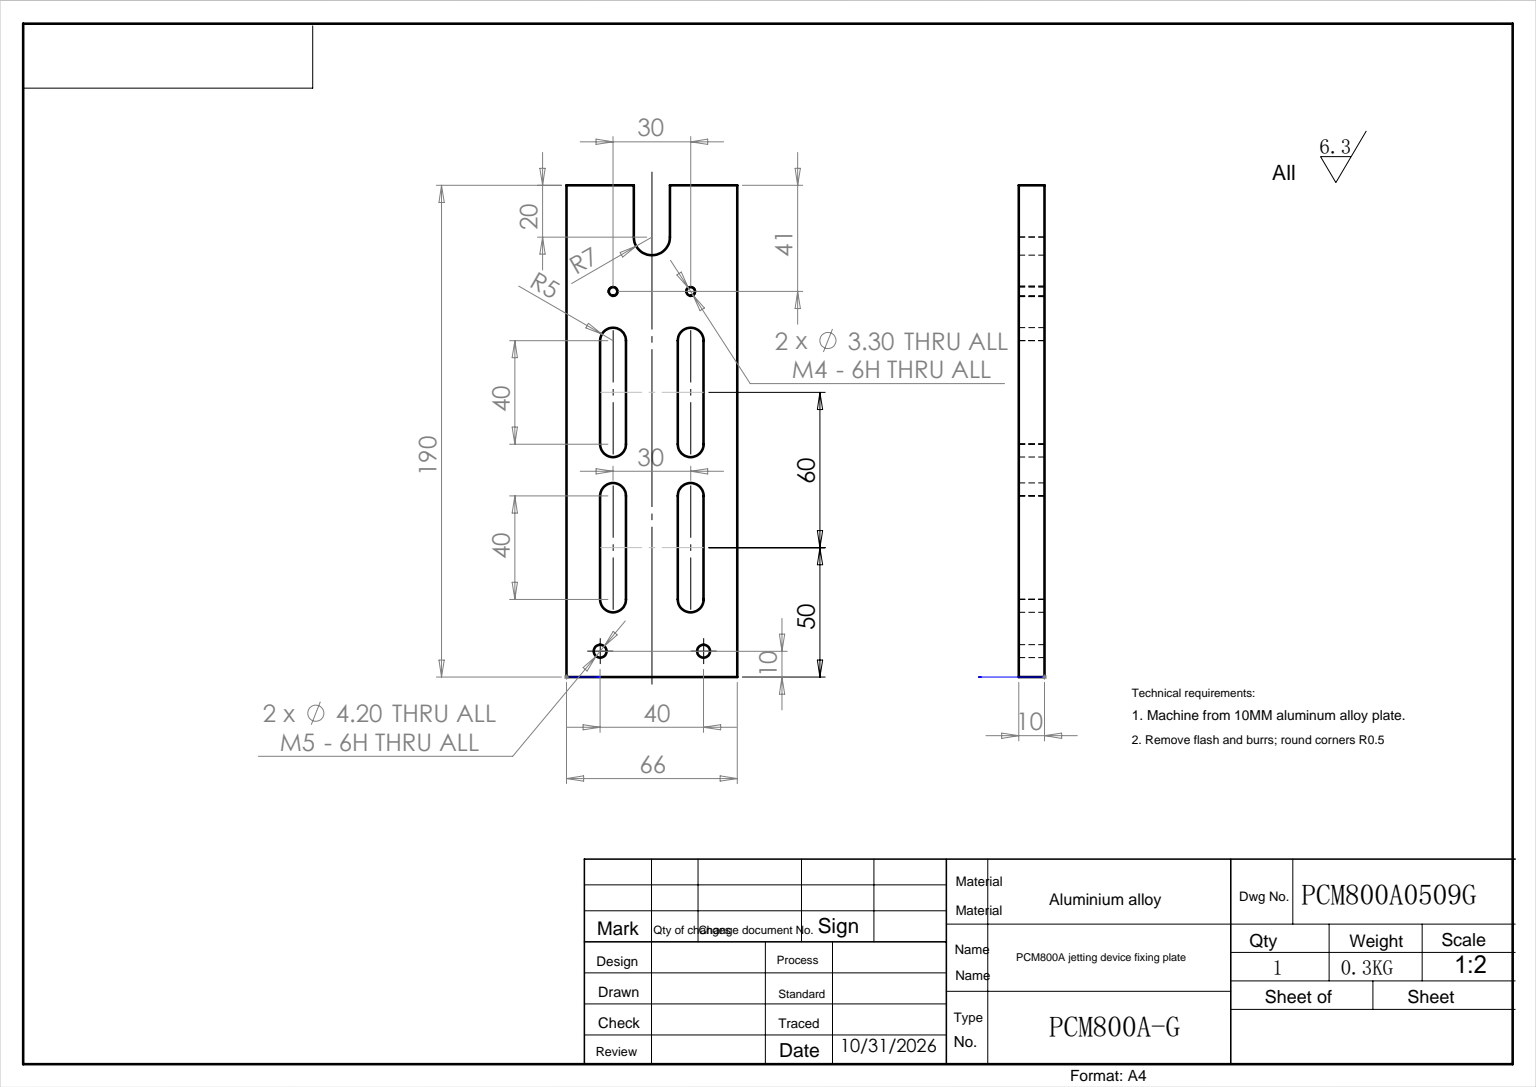
SolidWorks part; units mm, degrees
ref_plane "前视" through (0, 0, 0) normal (0, 0, 1) x (1, 0, 0)
ref_plane "上视" through (0, 0, 0) normal (0, 1, 0) x (1, 0, 0)
ref_plane "右视" through (0, 0, 0) normal (1, 0, 0) x (0, 0, -1)
sketch "草图1" plane through (0, 0, 0) normal (0, 0, 1) x (1, 0, 0)
  line L1 (0, 0) -> (66, 0)
  line L2 (0, 0) -> (0, 10)
  line L3 (0, 10) -> (66, 10)
  line L4 (66, 0) -> (66, 10)
  dimension "D1" = 66
  dimension "D2" = 10
extrude "拉伸1" add sketch "草图1" along normal blind 190
sketch "草图5" plane through (0, 10, 0) normal (0, 1, 0) x (-1, 0, 0)
  line L0 (-33, 0) -> (-33, 214.8788) construction
  line L1 (-66, 0) -> (0, 0) construction
  line L2 (-48, -4.4893) -> (-48, 82.7828) construction
  line L3 (-43, 70) -> (-43, 30)
  line L4 (-53, 70) -> (-53, 30)
  line L5 (-13, 70) -> (-13, 30)
  line L6 (-23, 70) -> (-23, 30)
  line L7 (-43, 130) -> (-43, 90)
  line L8 (-53, 130) -> (-53, 90)
  line L9 (-13, 130) -> (-13, 90)
  line L10 (-23, 130) -> (-23, 90)
  arc A0 (-53, 30) -> (-43, 30) centre (-48, 30) ccw
  arc A1 (-43, 70) -> (-53, 70) centre (-48, 70) ccw
  arc A2 (-23, 70) -> (-13, 70) centre (-18, 70) cw
  arc A3 (-13, 30) -> (-23, 30) centre (-18, 30) cw
  arc A4 (-53, 90) -> (-43, 90) centre (-48, 90) ccw
  arc A5 (-43, 130) -> (-53, 130) centre (-48, 130) ccw
  arc A6 (-23, 130) -> (-13, 130) centre (-18, 130) cw
  arc A7 (-13, 90) -> (-23, 90) centre (-18, 90) cw
  dimension "D2" = 10
  dimension "D3" = 10
  dimension "D1" = 15
  dimension "D4" = 30
  dimension "D5" = 40
  dimension "D6" = 2
extrude "切除-拉伸2" cut sketch "草图5" against normal through all
ref_plane "基准面1" through (33, 0, 0) normal (1, 0, 0) x (0, 0, -1)
hole_wizard "M5 螺纹孔1" positions "草图7" profile "草图8" tap size "M5" standard "GB" end condition through all
sketch "草图7" plane through (0, 10, 0) normal (0, 1, 0) x (-1, 0, 0)
  line L0 (-72.1814, 10) -> (9.6512, 10) construction
  line L1 (-66, 0) -> (0, 0) construction
  line L2 (-33, 0) -> (-33, 30.1795) construction
  point P0 (-13, 10)
  point P7 (-53, 10)
  dimension "D1" = 10
  dimension "D2" = 20
sketch "草图8" plane through (13, 10, 10) normal (1, 0, 0) x (0, 0, 1)
  line L0 (0, 0) -> (0, 10)
  line L1 (0, 10) -> (2.5, 10)
  line L2 (2.5, 10) -> (2.5, 0)
  line L5 (2.5, 0) -> (0, 0)
  line L11 (0, -6.35) -> (0, 107.95) construction
  dimension "螺纹线主直径" = 5
  dimension "通孔螺纹孔钻头深度" = 10
sketch "草图11" plane through (0, 10, 0) normal (0, 1, 0) x (-1, 0, 0)
  line L0 (-33, 190) -> (-33, 0) construction
  line L1 (-66, 190) -> (0, 190) construction
  line L2 (-66, 0) -> (0, 0) construction
  line L3 (-40, 249.7508) -> (-40, 170)
  line L4 (-26, 249.7508) -> (-26, 170)
  line L5 (-40, 249.7508) -> (-26, 249.7508)
  arc A0 (-40, 170) -> (-26, 170) centre (-33, 170) ccw
  dimension "D1" = 14
  dimension "D2" = 20
extrude "切除-拉伸3" cut sketch "草图11" against normal through all
hole_wizard "M4 螺纹孔1" positions "草图13" profile "草图12" tap size "M4" standard "GB" end condition through all
sketch "草图13" plane through (0, 0, 0) normal (0, -1, 0) x (1, 0, 0)
  line L0 (18, 149) -> (85.083, 149) construction
  line L2 (33, 170) -> (33, 74.4948) construction
  line L4 (40, 190) -> (66, 190) construction
  point P0 (18, 149)
  point P1 (48, 149)
  dimension "D1" = 15
  dimension "D2" = 30
  dimension "D3" = 41
sketch "草图12" plane through (18, 0, 149) normal (1, 0, 0) x (0, 0, -1)
  line L0 (0, 0) -> (0, 10)
  line L1 (0, 10) -> (1.65, 10)
  line L2 (1.65, 10) -> (1.65, 0)
  line L5 (1.65, 0) -> (0, 0)
  line L11 (0, -6.35) -> (0, 107.95) construction
  dimension "通孔螺纹孔钻头直径" = 3.3
  dimension "通孔螺纹孔钻头深度" = 10
cosmetic thread "孔螺蚊线1" parameters "D2"=4
cosmetic thread "孔螺蚊线2" parameters "D2"=4
